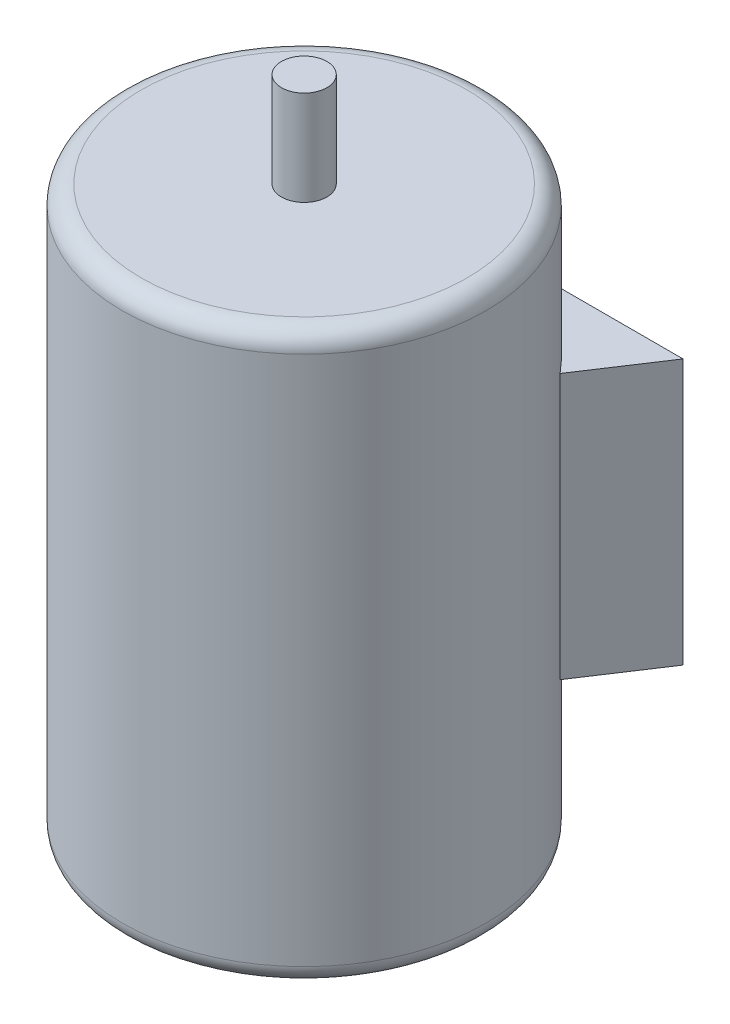
from build123d import *

# Parameters (mm, degrees)
SKETCH1_R           = 96
BOSS_EXTRUDE1_DEPTH = 300
SKETCH2_R           = 12
BOSS_EXTRUDE2_DEPTH = 50
FILLET1_R           = 10
BOSS_EXTRUDE3_DEPTH = 140


with BuildPart() as part:
    # Sketch1 → Boss-Extrude1 (new body)
    with BuildSketch(Plane(origin=(0, 0, 0), x_dir=(1, 0, 0), z_dir=(0, 1, 0))):
        with Locations(Location((0, 0, 0), (0, 0, 270))):
            Circle(SKETCH1_R)
    extrude(amount=BOSS_EXTRUDE1_DEPTH)

    # Sketch2 → Boss-Extrude2 (add)
    with BuildSketch(Plane(origin=(0, 300, 0), x_dir=(1, 0, 0), z_dir=(0, 1, 0))):
        with Locations(Location((0, 0, 0), (0, 0, 270))):
            Circle(SKETCH2_R)
    extrude(amount=BOSS_EXTRUDE2_DEPTH)

    # Fillet1
    fillet1_edges = [part.edges().sort_by_distance(p)[0] for p in [
        (0, 0, -96),
        (0, 300, -96),
    ]]
    fillet(fillet1_edges, radius=FILLET1_R)

    # Sketch3 → Boss-Extrude3 (add)
    with BuildSketch(Plane(origin=(0, 80, 0), x_dir=(-1, 0, 0), z_dir=(0, -1, 0))):
        with BuildLine():
            Line((74.225483886, 60.881668357), (100, 100))
            Line((100, 100), (-100, 100))
            Line((-100, 100), (-74.225483886, 60.881668357))
            ThreePointArc((-74.225483886, 60.881668357), (0, 96), (74.225483886, 60.881668357))
        make_face()
    extrude(amount=-BOSS_EXTRUDE3_DEPTH)


solid = part.part
